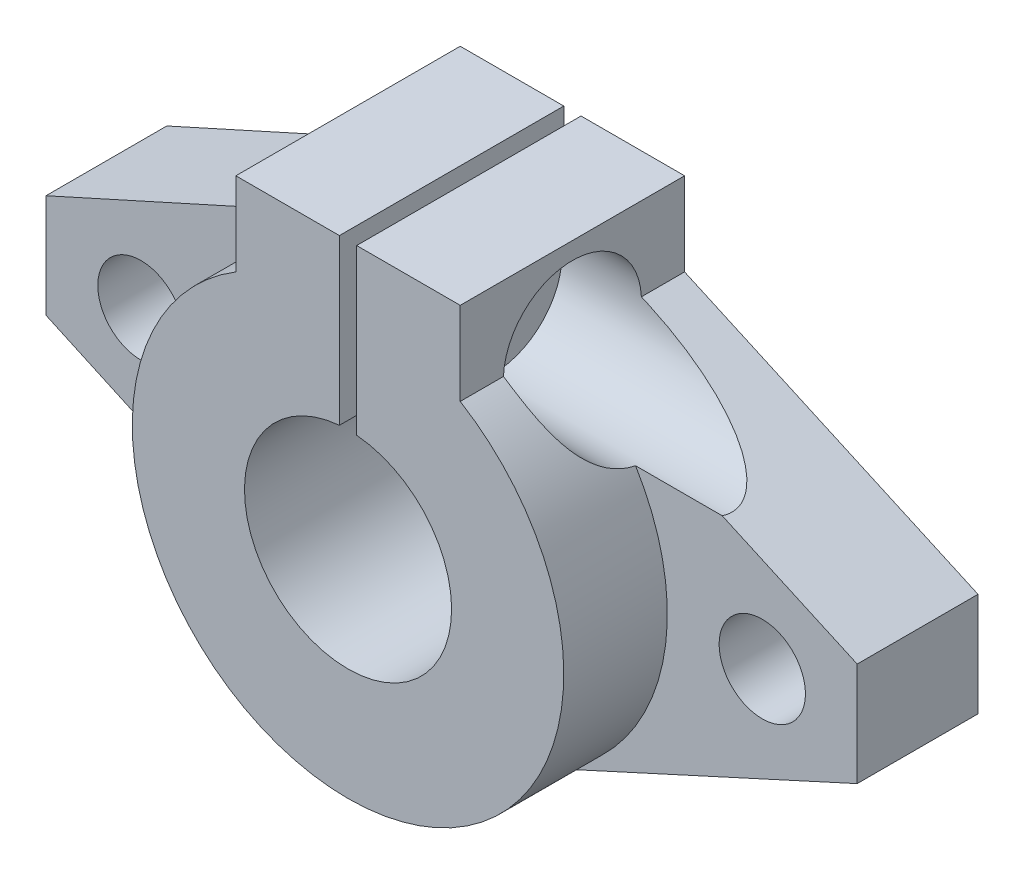
from build123d import *
from build123d.topology import SkipClean

# Parameters (mm, degrees)
EXTRUDE_1_DEPTH     = 6.5
EXTRUDE_START       = -7
SKETCH_2_R          = 2.5
EXTRUDE_2_DEPTH     = 7
SKETCH_3_W          = 1.65
SKETCH_3_H          = 23
CUT_EXTRUDE_START   = 10
CUT_EXTRUDE_1_DEPTH = 10


with BuildPart() as part:
    # 草图1 → 凸台-拉伸1 (new, symmetric)
    with BuildSketch(Plane.XY):
        with BuildLine():
            Line((0.5, 5.979130372), (0.5, 15.5))
            Line((0.5, 15.5), (6.5, 15.5))
            Line((6.5, 15.5), (6.5, 10.677078252))
            ThreePointArc((6.5, 10.677078252), (0, -12.5), (-6.5, 10.677078252))
            Line((-6.5, 10.677078252), (-6.5, 15.5))
            Line((-6.5, 15.5), (-0.5, 15.5))
            Line((-0.5, 15.5), (-0.5, 5.979130372))
            ThreePointArc((-0.5, 5.979130372), (0, -6), (0.5, 5.979130372))
        make_face()
    extrude(amount=EXTRUDE_1_DEPTH, both=True)

    # 草图2 → 凸台-拉伸2 (add)
    # profile 1 of 2: a face of its own
    with BuildSketch(Plane(origin=(0, 0, -6.5), x_dir=(-1, 0, 0), z_dir=(0, 0, -1)).offset(EXTRUDE_START)):
        with BuildLine():
            Line((-23.5, -3), (-5.197687408, -11.368115306))
            ThreePointArc((-5.197687408, -11.368115306), (-12.478245567, -0.737148272), (-6.5, 10.677078252))
            Line((-6.5, 10.677078252), (-23.5, 3))
            Line((-23.5, 3), (-23.5, -3))
        make_face()
        with Locations((-18, 0)):
            Circle(SKETCH_2_R, mode=Mode.SUBTRACT)
    # profile 2 of 2: a face of its own
    with BuildSketch(Plane(origin=(0, 0, -6.5), x_dir=(-1, 0, 0), z_dir=(0, 0, -1)).offset(EXTRUDE_START)):
        with BuildLine():
            ThreePointArc((6.5, 10.677078252), (12.478245567, -0.737148272), (5.197687408, -11.368115306))
            Line((5.197687408, -11.368115306), (23.5, -3))
            Line((23.5, -3), (23.5, 3))
            Line((23.5, 3), (6.5, 10.677078252))
        make_face()
        with Locations((18, 0)):
            Circle(SKETCH_2_R, mode=Mode.SUBTRACT)
    extrude(amount=EXTRUDE_2_DEPTH)

    # 草图3 → M4 螺纹孔1 (revolve, cut)
    with BuildSketch(Plane(origin=(-0.5, 11.5, 0), x_dir=(0, 0, -1), z_dir=(0, 1, 0))):
        with Locations((0.825, 11.5)):
            Rectangle(SKETCH_3_W, SKETCH_3_H)
    revolve(axis=Axis((5.85, 11.5, 0), (-1, 0, 0)), mode=Mode.SUBTRACT)

    # 草图5 → 打孔尺寸(%根据)内六角圆柱头螺钉的类型1 (revolve, cut)
    with BuildSketch(Plane(origin=(6.5, 10.5, 0), x_dir=(0, 0, -1), z_dir=(0, 1, 0))):
        Polygon((0, 0), (0, 7.351936393), (2.25, 6), (2.25, 4.6), (4, 4.6), (4, 0), align=None)
    revolve(axis=Axis((12.85, 10.5, 0), (-1, 0, 0)), mode=Mode.SUBTRACT)

    # 草图7 → 切除-拉伸1 (cut)
    with SkipClean():  # the faces are left unmerged after this step: merging them gives an invalid solid
        with BuildSketch(Plane(origin=(6.5, 0, 0), x_dir=(0, 0, -1), z_dir=(1, 0, 0)).offset(CUT_EXTRUDE_START)):
            with BuildLine():
                Line((-0.5, 10.677078252), (-3.996078489, 10.677078252))
                ThreePointArc((-3.996078489, 10.677078252), (0, 6.5), (3.996078489, 10.677078252))
                Line((3.996078489, 10.677078252), (-0.5, 10.677078252))
            make_face()
        extrude(amount=-CUT_EXTRUDE_1_DEPTH, mode=Mode.SUBTRACT)


solid = part.part
